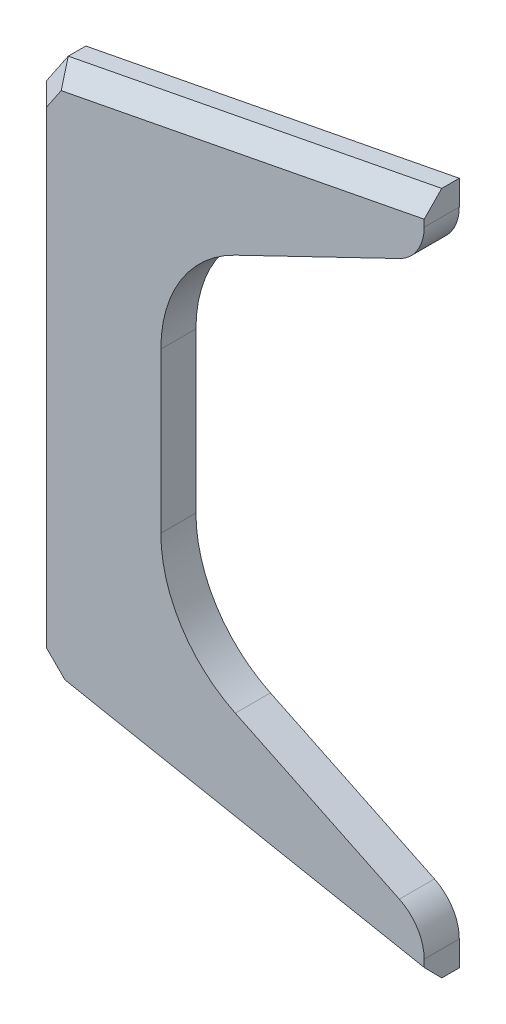
SolidWorks part; units mm, degrees
ref_plane "Front Plane" through (0, 0, 0) normal (0, 0, 1) x (1, 0, 0)
ref_plane "Top Plane" through (0, 0, 0) normal (0, 1, 0) x (1, 0, 0)
ref_plane "Right Plane" through (0, 0, 0) normal (1, 0, 0) x (0, 0, -1)
sketch "Sketch1" plane through (0, 0, 0) normal (0, 0, 1) x (1, 0, 0)
  line L0 (0, -121) -> (0, 121)
  line L1 (0, 121) -> (180, 155.8)
  line L2 (180, 155.8) -> (180, 144.471)
  line L3 (168.6864, 126.4558) -> (93.9407, 90.4153)
  line L4 (60, 36.3699) -> (60, -36.2699)
  line L5 (93.9407, -90.3153) -> (168.6864, -126.3558)
  line L6 (180, -144.371) -> (180, -155.8)
  line L7 (180, -155.8) -> (0, -121)
  line L8 (0, 0) -> (81.9386, 0) construction
  arc A0 (180, -144.371) -> (168.6864, -126.3558) centre (160, -144.371) ccw
  arc A1 (180, 144.471) -> (168.6864, 126.4558) centre (160, 144.471) cw
  arc A2 (93.9407, -90.3153) -> (60, -36.2699) centre (120, -36.2699) cw
  arc A3 (60, 36.3699) -> (93.9407, 90.4153) centre (120, 36.3699) cw
  point P17 (60, -73.95)
  point P20 (60, 74.05)
  dimension "D12" = 20
  dimension "D13" = 60
  dimension "D1" = 60
  dimension "D2" = 242
  dimension "D3" = 242
  dimension "D4" = 311.6
  dimension "D5" = 311.6
  dimension "D6" = 180
  dimension "D7" = 180
  dimension "D8" = 148.1
  dimension "D9" = 148
  dimension "D10" = 14.8
  dimension "D11" = 14.8
extrude "Boss-Extrude1" add sketch "Sketch1" along normal blind 16
chamfer "Chamfer1" distance 10 angle 45 2 edges at (0, 121, 8) (0, -121, 8)
chamfer "Chamfer2" distance 8 angle 45 5 edges at (94.9091, 139.3491, 16) (4.9091, 115.636, 16) (6.1983, -117.1983, 16) (96.1983, -139.5983, 16) (0, -1.3131, 16)
